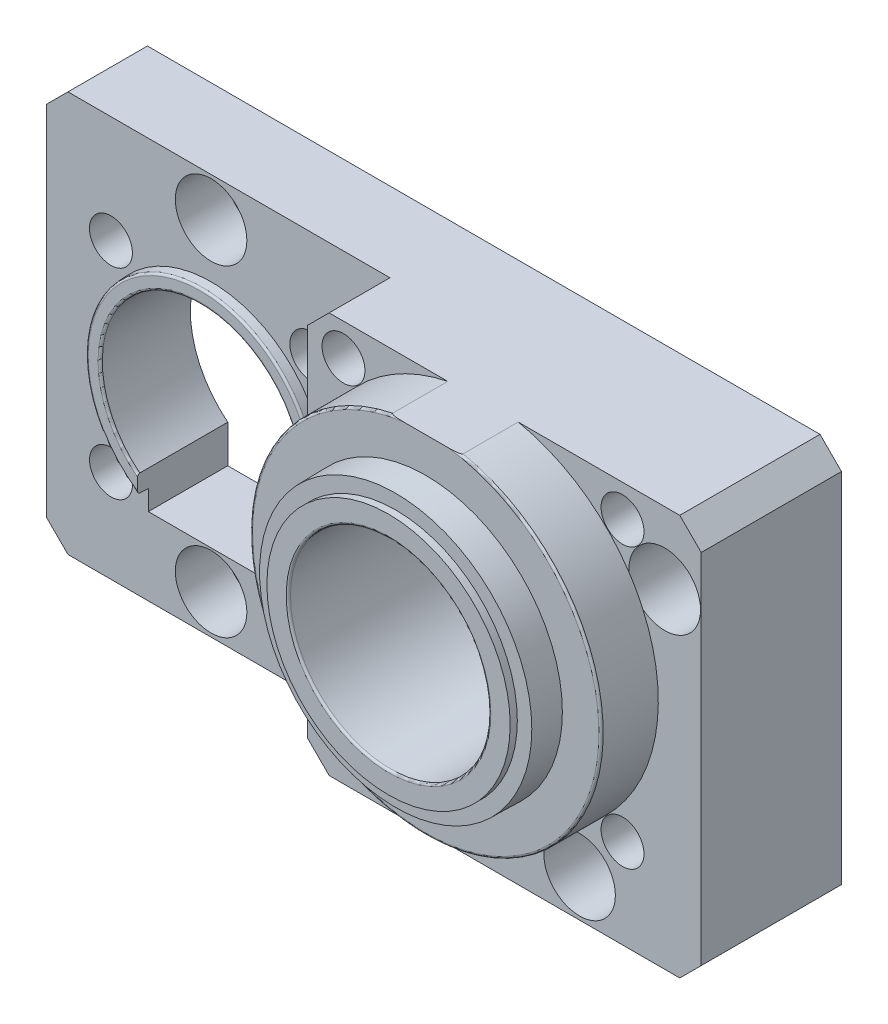
from build123d import *

# Parameters (mm, degrees)
SKETCH1_W                                    = 100
SKETCH1_H                                    = 56
BOSS_EXTRUDE1_DEPTH                          = 27.6
SKETCH2_R                                    = 19.095
BOSS_EXTRUDE2_DEPTH                          = 5.2
BOSS_EXTRUDE2_TAPER                          = 1
SKETCH4_W                                    = 117.356631531
SKETCH4_H                                    = 93.478875332
SKETCH4_R                                    = 24.5
CUT_EXTRUDE1_DEPTH                           = 8
FILLET1_R                                    = 0.3
SKETCH5_W                                    = 56.36290192
SKETCH5_H                                    = 22.991022885
CUT_EXTRUDE2_DEPTH                           = 97.914526075
SKETCH6_R                                    = 16.02
BOSS_EXTRUDE3_DEPTH                          = 1.5
BOSS_EXTRUDE3_TAPER                          = 2.8
FILLET2_R                                    = 0.3
CUT_EXTRUDE3_DEPTH                           = 90.406696404
CUT_EXTRUDE3_DEPTH_BACK                      = 90.406696404
SKETCH7_R                                    = 3
SKETCH8_R                                    = 14
CUT_EXTRUDE4_DEPTH                           = 90.054519041
SKETCH9_W                                    = 17.539210826
SKETCH9_H                                    = 13.762480841
CUT_EXTRUDE5_DEPTH                           = 93.728136852
CHAMFER1_SIZE                                = 3
CBORE_FOR_M6_HEX_SOCKET_HEAD_CAP_SCR_2_COUNT = 2
CBORE_FOR_M6_HEX_SOCKET_HEAD_CAP_SCR_2_PITCH = 75.00036
CBORE_FOR_M6_HEX_SOCKET_HEAD_CAP_SCR_3_COUNT = 2
CBORE_FOR_M6_HEX_SOCKET_HEAD_CAP_SCR_3_PITCH = 45
CBORE_FOR_M6_HEX_SOCKET_HEAD_CAP_SCR_4_COUNT = 2
CBORE_FOR_M6_HEX_SOCKET_HEAD_CAP_SCR_4_PITCH = 72.041132072
SKETCH12_R                                   = 14
CUT_EXTRUDE6_DEPTH                           = 93.728136852
FILLET3_R                                    = 0.3
SKETCH13_R                                   = 21.226121865
SKETCH13_R_2                                 = 17
CUT_EXTRUDE7_DEPTH                           = 1


with BuildPart() as part:
    # Sketch1 → Boss-Extrude1 (new body)
    with BuildSketch(Plane.XY):
        with Locations((-21.976283301, 20.395061728)):
            Rectangle(SKETCH1_W, SKETCH1_H)
    extrude(amount=BOSS_EXTRUDE1_DEPTH)

    # Sketch2 → Boss-Extrude2 (add)
    with BuildSketch(Plane.XY.offset(27.6)):
        with Locations((-2.477895801, 24.394261729)):
            Circle(SKETCH2_R)
    extrude(amount=BOSS_EXTRUDE2_DEPTH, taper=BOSS_EXTRUDE2_TAPER)

    # Sketch4 → Cut-Extrude1 (cut)
    with BuildSketch(Plane.XY.offset(27.6)):
        with Locations((-19.266750683, 19.548332785)):
            Rectangle(SKETCH4_W, SKETCH4_H)
        with Locations((-2.477895801, 24.394261729)):
            Circle(SKETCH4_R, mode=Mode.SUBTRACT)
    extrude(amount=-CUT_EXTRUDE1_DEPTH, mode=Mode.SUBTRACT)

    # Fillet1
    fillet1_edges = [part.edges().sort_by_distance(p)[0] for p in [
        (-21.482129463, 24.394261729, 32.8),
    ]]
    fillet(fillet1_edges, radius=FILLET1_R)

    # Sketch5 → Cut-Extrude2 (cut, through all)
    with BuildSketch(Plane.XZ.offset(7.604938272)):
        with Locations((-55.159346761, 22.595511443)):
            Rectangle(SKETCH5_W, SKETCH5_H)
    extrude(amount=-CUT_EXTRUDE2_DEPTH, mode=Mode.SUBTRACT)

    # Sketch6 → Boss-Extrude3 (add)
    with BuildSketch(Plane.XY.offset(11.1)):
        with Locations((-48.976733301, 19.394386728)):
            Circle(SKETCH6_R)
    extrude(amount=BOSS_EXTRUDE3_DEPTH, taper=BOSS_EXTRUDE3_TAPER)

    # Fillet2
    fillet2_edges = [part.edges().sort_by_distance(p)[0] for p in [
        (-64.923371062, 19.394386728, 12.6),
    ]]
    fillet(fillet2_edges, radius=FILLET2_R)

    # Sketch7 → Cut-Extrude3 (cut, two sides: drawn at the far end of the back side and taken through both)
    with BuildSketch(Plane.XY.offset(11.1).offset(-CUT_EXTRUDE3_DEPTH_BACK)):
        with Locations((-62.976383301, 33.394036728)):
            Circle(SKETCH7_R)
        with Locations((-34.977083301, 5.394736728)):
            Circle(SKETCH7_R)
        with Locations((-62.959232869, 5.377309322)):
            Circle(SKETCH7_R)
        with Locations((-34.977083301, 33.394036728)):
            Circle(SKETCH7_R)
        with Locations((-21.977408301, 4.894749229)):
            Circle(SKETCH7_R)
        with Locations((17.021616699, 4.894749228)):
            Circle(SKETCH7_R)
        with Locations((-21.977408301, 43.893774228)):
            Circle(SKETCH7_R)
        with Locations((17.021616699, 43.893774228)):
            Circle(SKETCH7_R)
    extrude(amount=CUT_EXTRUDE3_DEPTH + CUT_EXTRUDE3_DEPTH_BACK, mode=Mode.SUBTRACT)

    # Sketch8 → Cut-Extrude4 (cut, through all)
    with BuildSketch(Plane.XY.offset(12.6)):
        with Locations((-48.976733301, 19.394386728)):
            Circle(SKETCH8_R)
    extrude(amount=-CUT_EXTRUDE4_DEPTH, mode=Mode.SUBTRACT)

    # Sketch9 → Cut-Extrude5 (cut, through all)
    with BuildSketch(Plane(origin=(0, 0, 0), x_dir=(-1, 0, 0), z_dir=(0, 0, -1))):
        with Locations((48.976733301, 10.086184236)):
            Rectangle(SKETCH9_W, SKETCH9_H)
    extrude(amount=-CUT_EXTRUDE5_DEPTH, mode=Mode.SUBTRACT)

    # Chamfer1
    chamfer1_edges = [part.edges().sort_by_distance(p)[0] for p in [
        (28.023716699, 48.395061728, 9.8),
        (28.023716699, -7.604938272, 9.8),
        (-71.976283301, 48.395061728, 5.55),
        (-71.976283301, -7.604938272, 5.55),
        (-26.977895801, -7.604938272, 15.35),
        (-26.977895801, 48.395061728, 15.35),
    ]]
    chamfer(chamfer1_edges, length=CHAMFER1_SIZE)

    # Sketch11 → CBORE for M6 Hex Socket Head Cap Screw1 (revolve, cut)
    with BuildSketch(Plane(origin=(-48.976733301, 42.895061728, 19.6), x_dir=(0, -1, 0), z_dir=(1, 0, 0))):
        Polygon((0, 0), (0, 19.6), (3.2, 19.6), (3.2, 15.5), (5, 15.5), (5, 0), align=None)
    cbore_for_m6_hex_socket_head_cap_screw1 = revolve(axis=Axis((-48.976733301, 42.895061728, 25.95), (0, 0, -1)), mode=Mode.SUBTRACT)

    # CBORE for M6 Hex Socket Head Cap Scr 2: CBORE for M6 Hex Socket Head Cap Screw1 ×2
    with Locations(*[Vector(0.8000021599844496, -0.5999971200099341, 0) * (i * CBORE_FOR_M6_HEX_SOCKET_HEAD_CAP_SCR_2_PITCH) for i in range(1, CBORE_FOR_M6_HEX_SOCKET_HEAD_CAP_SCR_2_COUNT)]):
        add(cbore_for_m6_hex_socket_head_cap_screw1, mode=Mode.SUBTRACT)

    # CBORE for M6 Hex Socket Head Cap Scr 3: CBORE for M6 Hex Socket Head Cap Screw1 ×2
    with Locations(*[(0, -i * CBORE_FOR_M6_HEX_SOCKET_HEAD_CAP_SCR_3_PITCH, 0) for i in range(1, CBORE_FOR_M6_HEX_SOCKET_HEAD_CAP_SCR_3_COUNT)]):
        add(cbore_for_m6_hex_socket_head_cap_screw1, mode=Mode.SUBTRACT)

    # CBORE for M6 Hex Socket Head Cap Scr 4: CBORE for M6 Hex Socket Head Cap Screw1 ×2
    with Locations(*[Vector(0.9980471979289498, -0.06246431546228526, 0) * (i * CBORE_FOR_M6_HEX_SOCKET_HEAD_CAP_SCR_4_PITCH) for i in range(1, CBORE_FOR_M6_HEX_SOCKET_HEAD_CAP_SCR_4_COUNT)]):
        add(cbore_for_m6_hex_socket_head_cap_screw1, mode=Mode.SUBTRACT)

    # Sketch12 → Cut-Extrude6 (cut, through all)
    with BuildSketch(Plane.XY.offset(32.8)):
        with Locations((-2.477895801, 24.394261729)):
            Circle(SKETCH12_R)
    extrude(amount=-CUT_EXTRUDE6_DEPTH, mode=Mode.SUBTRACT)

    # Fillet3
    fillet3_edges = [part.edges().sort_by_distance(p)[0] for p in [
        (-48.976733301, 33.394386728, 12.6),
        (-2.477895801, -0.105738271, 27.6),
        (-16.477895801, 24.394261729, 32.8),
    ]]
    fillet(fillet3_edges, radius=FILLET3_R)

    # Sketch13 → Cut-Extrude7 (cut)
    with BuildSketch(Plane.XY.offset(32.8)):
        with Locations((-2.477895801, 24.394261729)):
            Circle(SKETCH13_R)
        with Locations((-2.477895801, 24.394261729)):
            Circle(SKETCH13_R_2, mode=Mode.SUBTRACT)
    extrude(amount=-CUT_EXTRUDE7_DEPTH, mode=Mode.SUBTRACT)


solid = part.part
